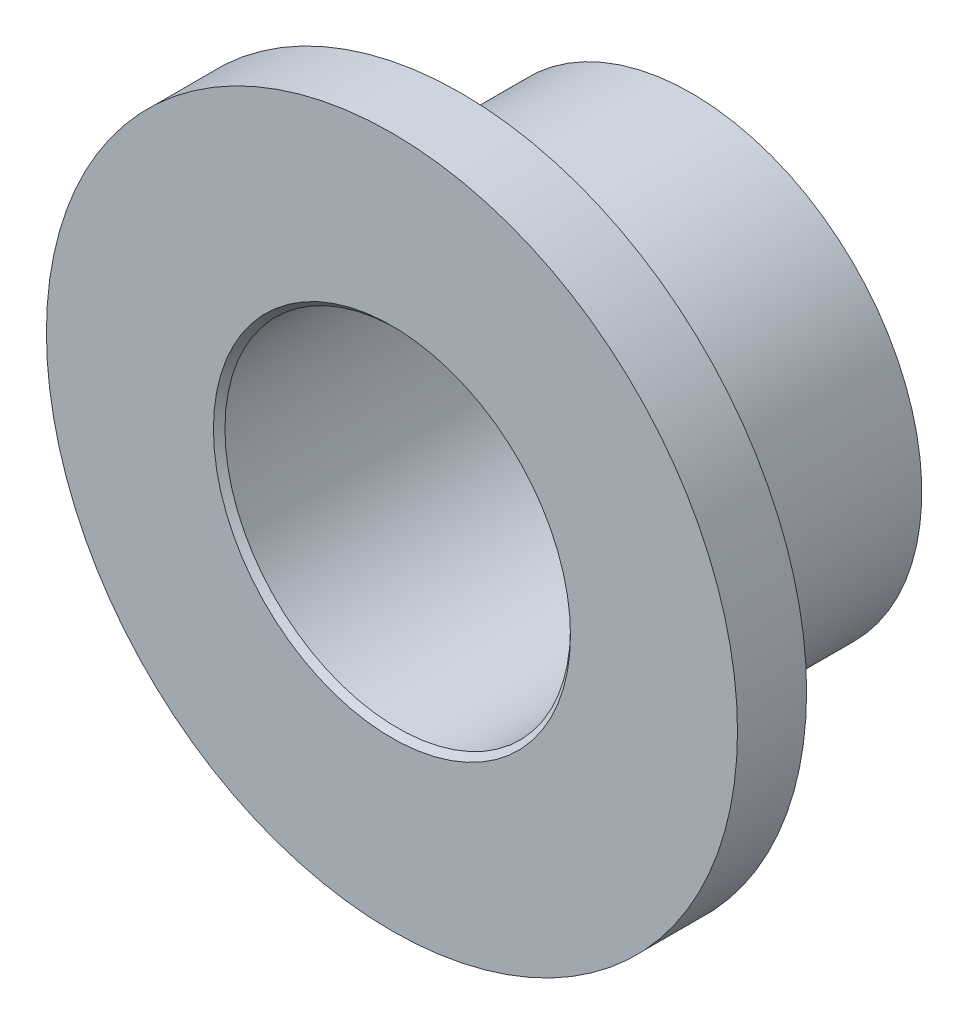
SolidWorks part; units mm, degrees
ref_plane "Front Plane" through (0, 0, 0) normal (0, 0, 1) x (1, 0, 0)
ref_plane "Top Plane" through (0, 0, 0) normal (0, 1, 0) x (1, 0, 0)
ref_plane "Right Plane" through (0, 0, 0) normal (1, 0, 0) x (0, 0, -1)
sketch "Sketch1" plane through (0, 0, 0) normal (0, 0, 1) x (1, 0, 0)
  circle A0 centre (0, 0) radius 20
  circle A2 centre (0, 0) radius 15
  dimension "D1" = 40
extrude "Boss-Extrude1" add sketch "Sketch1" along normal blind 26
sketch "Sketch2" plane through (0, 0, 26) normal (0, 0, 1) x (1, 0, 0)
  circle A0 centre (0, 0) radius 30
  circle A1 centre (0, 0) radius 15
  dimension "D1" = 60
extrude "Boss-Extrude2" add sketch "Sketch2" against normal blind 6
fillet "Fillet1" radius 3 1 edges at (20, 0, 20)
chamfer "Chamfer2" distance 0.5 angle 45 2 edges at (15, 0, 26) (15, 0, 0)
